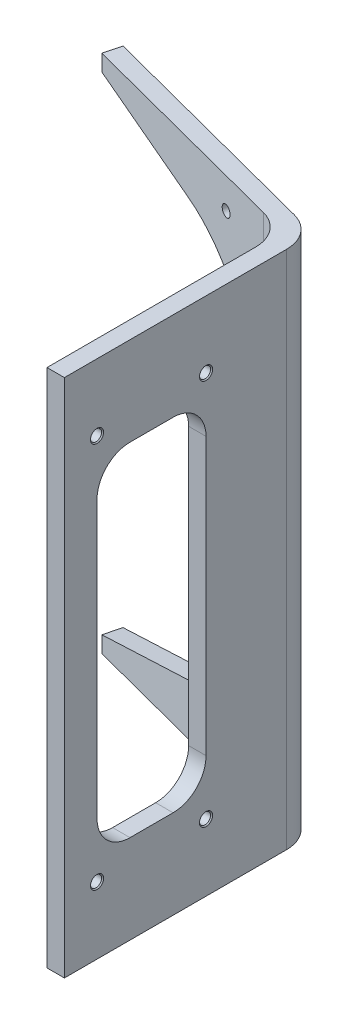
SolidWorks part; units mm, degrees
ref_plane "Front Plane" through (0, 0, 0) normal (0, 0, 1) x (1, 0, 0)
ref_plane "Top Plane" through (0, 0, 0) normal (0, 1, 0) x (1, 0, 0)
ref_plane "Right Plane" through (0, 0, 0) normal (1, 0, 0) x (0, 0, -1)
sketch "Sketch1" plane through (0, 0, 0) normal (0, 1, 0) x (1, 0, 0)
  line L0 (2489.7473, 1503.3882) -> (2505.7473, 1503.3882)
  line L1 (2489.7473, 1503.3882) -> (2489.7473, 1695.3302)
  line L2 (2465.8351, 1726.2913) -> (2264.6948, 1778.8341)
  line L3 (2268.7387, 1794.3146) -> (2264.6948, 1778.8341)
  line L4 (2505.7473, 1707.6875) -> (2505.7473, 1503.3882)
  line L5 (2481.8351, 1738.6486) -> (2268.7387, 1794.3146)
  arc A0 (2489.7473, 1695.3302) -> (2465.8351, 1726.2913) centre (2457.7473, 1695.3302) ccw
  arc A1 (2505.7473, 1707.6875) -> (2481.8351, 1738.6486) centre (2473.7473, 1707.6875) ccw
extrude "Boss-Extrude1" add sketch "Sketch1" along normal blind 478
sketch "Sketch2" plane through (2505.7473, 0, 0) normal (1, 0, 0) x (0, 0, -1)
  line L0 (1503.3882, 478) -> (1503.3882, 0) construction
  line L1 (1563.6882, 81.6) -> (1603.2882, 81.6)
  line L2 (1533.3882, 111.9) -> (1533.3882, 366.1)
  line L3 (1563.6882, 396.4) -> (1603.2882, 396.4)
  line L4 (1633.5882, 111.9) -> (1633.5882, 366.1)
  line L5 (1533.3882, 81.6) -> (1633.5882, 396.4) construction
  line L6 (1533.3882, 396.4) -> (1633.5882, 81.6) construction
  line L7 (1503.3882, 0) -> (1707.6875, 0) construction
  line L8 (1503.3882, 478) -> (1707.6875, 478) construction
  arc A0 (1563.6882, 81.6) -> (1533.3882, 111.9) centre (1563.6882, 111.9) cw
  arc A1 (1603.2882, 81.6) -> (1633.5882, 111.9) centre (1603.2882, 111.9) ccw
  arc A2 (1603.2882, 396.4) -> (1633.5882, 366.1) centre (1603.2882, 366.1) cw
  arc A3 (1533.3882, 366.1) -> (1563.6882, 396.4) centre (1563.6882, 366.1) cw
  point P0 (1583.4882, 239)
  dimension "D4" = 30.3
  dimension "D1" = 30
  dimension "D2" = 81.6
  dimension "D3" = 81.6
  dimension "D5" = 100.2
extrude "Cut-Extrude1" cut sketch "Sketch2" against normal blind 478
hole_wizard "M12 Tapped Hole1" positions "Sketch5" profile "Sketch6" tap size "M12" standard "GB" end condition through all
sketch "Sketch5" plane through (2505.7473, 0, 0) normal (1, 0, 0) x (0, 0, -1)
  line L5 (1533.3882, 61.45) -> (1633.5882, 61.45) construction
  line L6 (1533.3882, 61.45) -> (1533.3882, 416.55) construction
  line L7 (1533.3882, 416.55) -> (1633.5882, 416.55) construction
  line L8 (1633.5882, 61.45) -> (1633.5882, 416.55) construction
  point P10 (1633.5882, 416.55)
  point P53 (1533.3882, 61.45)
  point P54 (1533.3882, 416.55)
  point P55 (1633.5882, 61.45)
  dimension "D1" = 100.2
  dimension "D2" = 355.1
sketch "Sketch6" plane through (2505.7473, 416.55, -1633.5882) normal (0, 1, 0) x (0, 0, -1)
  line L0 (0, 0) -> (0, 241.0525)
  line L1 (0, 241.0525) -> (5.1, 241.0525)
  line L2 (5.1, 241.0525) -> (5.1, 0.925)
  line L3 (5.1, 0.925) -> (6.025, 0)
  line L5 (6.025, 0) -> (0, 0)
  line L6 (-5.1, 0.925) -> (-6.025, 0) construction
  line L11 (0, -6.35) -> (0, 107.95) construction
  dimension "通孔螺纹孔钻头直径" = 10.2
  dimension "通孔螺纹孔钻头深度" = 241.0525
  dimension "近端锥形沉头孔直径" = 12.05
  dimension "近端锥形沉头孔角度" = 90
cosmetic thread "Cosmetic thread 1" parameters "D2"=12
cosmetic thread "Cosmetic thread 2" parameters "D2"=12
cosmetic thread "Cosmetic thread 3" parameters "D2"=12
cosmetic thread "Cosmetic thread 4" parameters "D2"=12
sketch "Sketch7" plane through (583.7028, 0, -2234.4873) normal (0.2527, 0, -0.9675) x (-0.9675, 0, -0.2527)
  line L0 (-1741.5792, 463) -> (-1741.5792, 15)
  line L1 (-1741.5792, 478) -> (-1741.5792, 0) construction
  line L2 (-1741.5792, 15) -> (-1853.0788, 46.972)
  line L3 (-1932.1792, 151.9418) -> (-1932.1792, 326.0582)
  line L4 (-1853.0788, 431.028) -> (-1741.5792, 463)
  arc A0 (-1853.0788, 46.972) -> (-1932.1792, 151.9418) centre (-1822.9792, 151.9418) cw
  arc A1 (-1932.1792, 326.0582) -> (-1853.0788, 431.028) centre (-1822.9792, 326.0582) cw
  dimension "D6" = 109.2
  dimension "D1" = 448
  dimension "D2" = 15
  dimension "D3" = 106
  dimension "D4" = 106
  dimension "D5" = 190.6
extrude "Cut-Extrude2" cut sketch "Sketch7" against normal blind 478
hole_wizard "M12 Tapped Hole2" positions "Sketch9" profile "Sketch10" tap size "M12" standard "GB" end condition through all
sketch "Sketch9" plane through (583.7028, 0, -2234.4873) normal (0.2527, 0, -0.9675) x (-0.9675, 0, -0.2527)
  line L0 (-1741.5792, 478) -> (-1741.5792, 463) construction
  line L1 (-1741.5792, 15) -> (-1741.5792, 0) construction
  line L3 (-1961.8262, 478) -> (-1741.5792, 478) construction
  point P0 (-1901.4792, 450)
  point P2 (-1901.4792, 28)
  dimension "D1" = 159.9
  dimension "D2" = 159.9
  dimension "D3" = 422
  dimension "D4" = 28
sketch "Sketch10" plane through (2423.4473, 450, -1753.9009) normal (0, 1, 0) x (-0.9675, 0, -0.2527)
  line L0 (0, 0) -> (0, 282.503)
  line L1 (0, 282.503) -> (5.1, 282.503)
  line L2 (5.1, 282.503) -> (5.1, 0.925)
  line L3 (5.1, 0.925) -> (6.025, 0)
  line L5 (6.025, 0) -> (0, 0)
  line L6 (-5.1, 0.925) -> (-6.025, 0) construction
  line L11 (0, -6.35) -> (0, 107.95) construction
  dimension "通孔螺纹孔钻头直径" = 10.2
  dimension "通孔螺纹孔钻头深度" = 282.503
  dimension "近端锥形沉头孔直径" = 12.05
  dimension "近端锥形沉头孔角度" = 90
cosmetic thread "Cosmetic thread 5" parameters "D2"=12
cosmetic thread "Cosmetic thread 6" parameters "D2"=12
